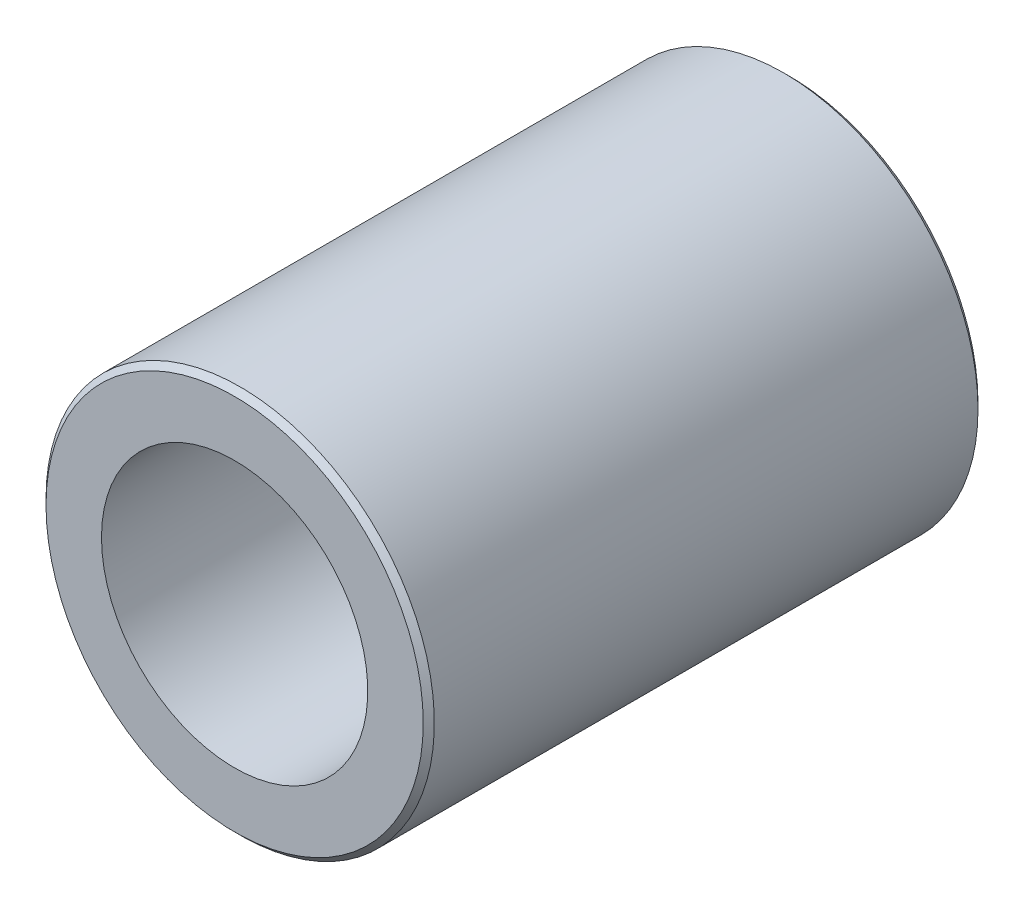
SolidWorks part; units mm, degrees
ref_plane "Front Plane" through (0, 0, 0) normal (0, 0, 1) x (1, 0, 0)
ref_plane "Top Plane" through (0, 0, 0) normal (0, 1, 0) x (1, 0, 0)
ref_plane "Right Plane" through (0, 0, 0) normal (1, 0, 0) x (0, 0, -1)
other "Configuration Table"
ref_plane "Plane1" through (0, 0, 0) normal (0, -1, 0) x (1, 0, 0)
sketch "Sketch1" plane through (0, 0, 0) normal (0, -1, 0) x (1, 0, 0)
  line L0 (12, 28) -> (12.5, 28)
  line L1 (12.5, 28) -> (12.5, 0)
  line L2 (12.5, 0) -> (17, 0)
  line L3 (17, 0) -> (17.5, 0.5)
  line L4 (17.5, 0.5) -> (17.5, 49.5)
  line L5 (17.5, 49.5) -> (17, 50)
  line L6 (17, 50) -> (12, 50)
  line L7 (12, 50) -> (12, 28)
  line L8 (0, 50) -> (0, 0) construction
revolve "Revolve1" add sketch "Sketch1" angle 360 about L8
